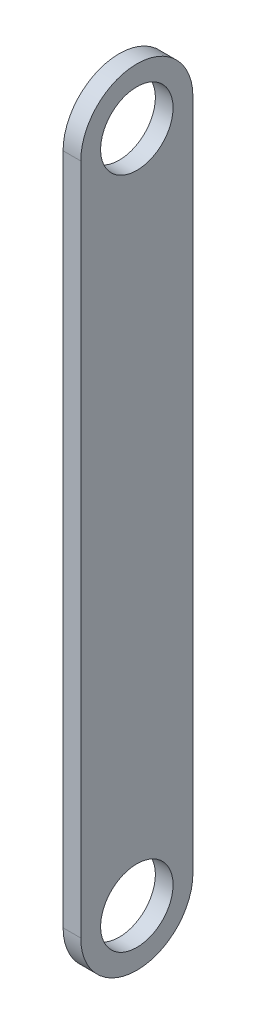
from build123d import *

# Parameters (mm, degrees)
SKETCH1_R           = 4.1
BOSS_EXTRUDE1_DEPTH = 2


with BuildPart() as part:
    # Sketch1 → Boss-Extrude1 (new body)
    with BuildSketch(Plane(origin=(0, 0, 0), x_dir=(0, 0, -1), z_dir=(1, 0, 0))):
        with BuildLine():
            Line((-6.35, -38.1), (-6.35, 38.1))
            ThreePointArc((-6.35, 38.1), (0, 44.45), (6.35, 38.1))
            Line((6.35, 38.1), (6.35, -38.1))
            ThreePointArc((6.35, -38.1), (0, -44.45), (-6.35, -38.1))
        make_face()
        with Locations((0, 38.1)):
            Circle(SKETCH1_R, mode=Mode.SUBTRACT)
        with Locations((0, -38.1)):
            Circle(SKETCH1_R, mode=Mode.SUBTRACT)
    extrude(amount=BOSS_EXTRUDE1_DEPTH)


solid = part.part
